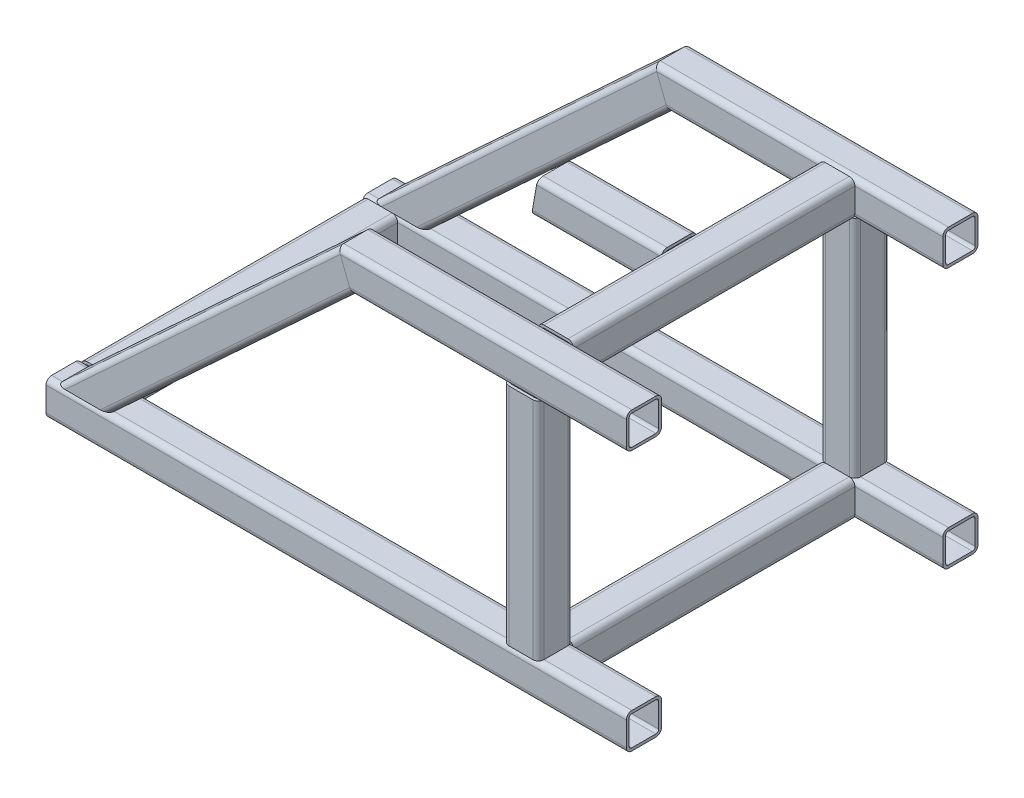
SolidWorks part; units mm, degrees
ref_plane "Front Plane" through (0, 0, 0) normal (0, 0, 1) x (1, 0, 0)
ref_plane "Top Plane" through (0, 0, 0) normal (0, 1, 0) x (1, 0, 0)
ref_plane "Right Plane" through (0, 0, 0) normal (1, 0, 0) x (0, 0, -1)
other "Configuration Table"
sketch3d "3DSketch1"
  line L0 (0, 0, 0) -> (0, 0, 450)
  line L1 (0, 0, 450) -> (0, 370, 450)
  line L2 (0, 0, 0) -> (0, 370, 0)
  line L3 (0, 370, 0) -> (0, 370, 450)
  line L4 (0, 0, 0) -> (-327.8919, 0, 0) construction
  line L5 (-650, 0, 0) -> (150, 0, 0)
  line L6 (0, 370, 0) -> (-264.4652, 370, 0) construction
  line L7 (0, 370, 450) -> (-208.2786, 370, 450) construction
  line L8 (0, 0, 450) -> (-224.2563, 0, 450) construction
  line L9 (-250, 370, 0) -> (150, 370, 0)
  line L10 (-650, 0, 450) -> (150, 0, 450)
  line L11 (-250, 370, 450) -> (150, 370, 450)
  line L13 (-650, 0, 0) -> (-650, 0, 450)
  line L16 (-250, 370, 0) -> (-650, 0, 0)
  line L17 (-250, 370, 450) -> (-650, 0, 450)
  line L18 (-250, 370, 450) -> (-250, 370, 0) construction
  line L19 (0, 370, 225) -> (-210, 370, 225)
other "Gb／6728-1986 square hollow section 050 X 50 X 4 (1)"
ref_plane "Plane1" through (-250, 370, 450) normal (1, 0, 0) x (0, 0, -1)
sketch "Sketch1" plane through (-250, 370, 450) normal (1, 0, 0) x (0, 0, -1)
  line L0 (-17, -21) -> (17, -21)
  line L1 (-21, -17) -> (-21, 17)
  line L2 (17, 21) -> (-17, 21)
  line L3 (21, 17) -> (21, -17)
  line L4 (-17, -25) -> (17, -25)
  line L5 (-25, -17) -> (-25, 17)
  line L6 (17, 25) -> (-17, 25)
  line L7 (25, 17) -> (25, -17)
  arc A0 (25, 17) -> (17, 25) centre (17, 17) ccw
  arc A1 (17, -25) -> (25, -17) centre (17, -17) ccw
  arc A2 (-25, -17) -> (-17, -25) centre (-17, -17) ccw
  arc A3 (-17, 25) -> (-25, 17) centre (-17, 17) ccw
  arc A4 (-17, 21) -> (-21, 17) centre (-17, 17) ccw
  arc A5 (21, 17) -> (17, 21) centre (17, 17) ccw
  arc A6 (17, -21) -> (21, -17) centre (17, -17) ccw
  arc A7 (-21, -17) -> (-17, -21) centre (-17, -17) ccw
  point P0 (-25, 0)
  point P1 (25, 0)
  point P2 (0, 25)
  point P3 (0, -25)
  point P4 (0, 0)
  point P5 (-25, -25)
  point P6 (25, -25)
  point P7 (25, 25)
  point P8 (-25, 25)
  point P33 (0, 0)
  dimension "D1" = 8
  dimension "Thickness" = 4
  dimension "V_leg" = 50
other "Gb／6728-1986 square hollow section 050 X 50 X 4 (12)"
ref_plane "Plane2" through (-250, 370, 0) normal (-0.7341, -0.679, 0) x (0.679, -0.7341, 0)
sketch "Sketch11" plane through (-250, 370, 0) normal (-0.7341, -0.679, 0) x (0.679, -0.7341, 0)
  line L0 (-17, -21) -> (17, -21)
  line L1 (-21, -17) -> (-21, 17)
  line L2 (17, 21) -> (-17, 21)
  line L3 (21, 17) -> (21, -17)
  line L4 (-17, -25) -> (17, -25)
  line L5 (-25, -17) -> (-25, 17)
  line L6 (17, 25) -> (-17, 25)
  line L7 (25, 17) -> (25, -17)
  arc A0 (25, 17) -> (17, 25) centre (17, 17) ccw
  arc A1 (17, -25) -> (25, -17) centre (17, -17) ccw
  arc A2 (-25, -17) -> (-17, -25) centre (-17, -17) ccw
  arc A3 (-17, 25) -> (-25, 17) centre (-17, 17) ccw
  arc A4 (-17, 21) -> (-21, 17) centre (-17, 17) ccw
  arc A5 (21, 17) -> (17, 21) centre (17, 17) ccw
  arc A6 (17, -21) -> (21, -17) centre (17, -17) ccw
  arc A7 (-21, -17) -> (-17, -21) centre (-17, -17) ccw
  point P0 (-25, 0)
  point P1 (25, 0)
  point P2 (0, 25)
  point P3 (0, -25)
  point P4 (0, 0)
  point P5 (-25, -25)
  point P6 (25, -25)
  point P7 (25, 25)
  point P8 (-25, 25)
  point P33 (0, 0)
  dimension "D1" = 8
  dimension "Thickness" = 4
  dimension "V_leg" = 50
other "Trim/Extend 2"
other "Trim/Extend 3"
other "Trim/Extend 4"
sketch "Sketch3" plane through (0, 0, 200) normal (0, 0, -1) x (-1, 0, 0)
  line L0 (210, 353) -> (210, 387) construction
  line L1 (210, 345) -> (210, 395)
  line L3 (25, 345) -> (210, 345) construction
  line L4 (25, 345) -> (210, 345) construction
  line L6 (25, 395) -> (210, 395) construction
  line L7 (25, 395) -> (210, 395) construction
  line L8 (201.1837, 395) -> (210, 345)
  line L9 (210, 395) -> (201.1837, 395)
  dimension "D1" = 50
  dimension "D2" = 10
extrude "Cut-Extrude1" cut sketch "Sketch3" against normal up to next contours L9 L8 L1
equation "\"D5@3DSketch1\"=\"D4@3DSketch1\""
equation "\"D9@3DSketch1\"=\"D8@3DSketch1\""
equation "\"D7@3DSketch1\"=\"D6@3DSketch1\""
equation "\"D4@3DSketch1\"=\"D6@3DSketch1\""
